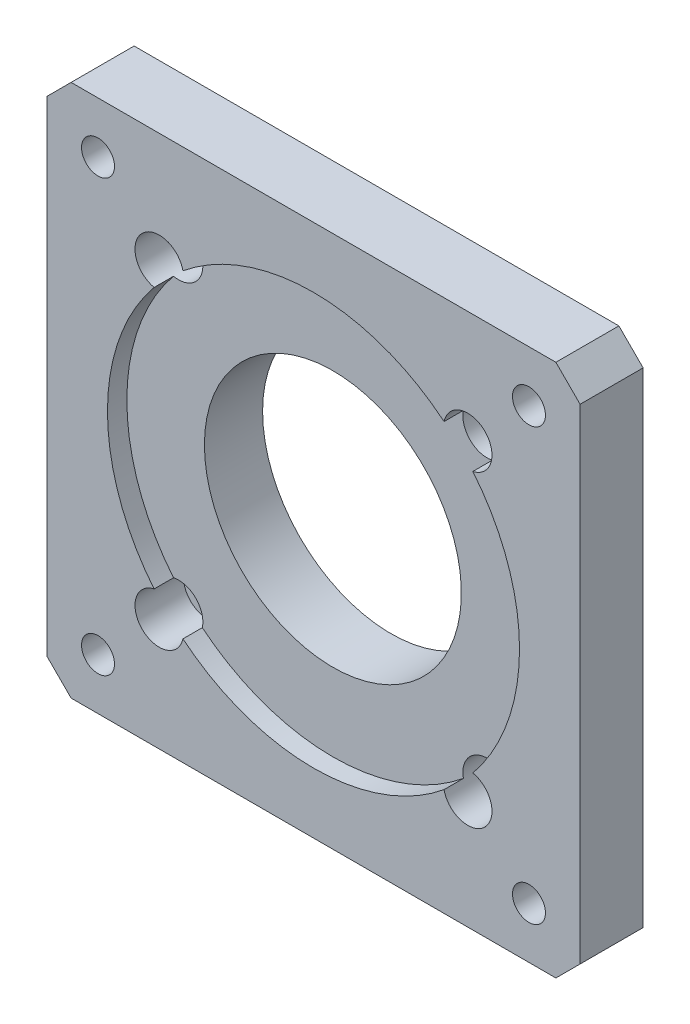
SolidWorks part; units mm, degrees
material "6061Al"
ref_plane "前视基准面" through (0, 0, 0) normal (0, 0, 1) x (1, 0, 0)
ref_plane "上视基准面" through (0, 0, 0) normal (0, 1, 0) x (1, 0, 0)
ref_plane "右视基准面" through (0, 0, 0) normal (1, 0, 0) x (0, 0, -1)
sketch "草图1" plane through (0, 0, 0) normal (0, 0, 1) x (1, 0, 0)
  line L1 (-55, 55) -> (55, 55)
  line L2 (-55, 55) -> (-55, -55)
  line L3 (-55, -55) -> (55, -55)
  line L4 (55, 55) -> (55, -55)
  line L5 (-55, 55) -> (55, -55) construction
  line L6 (-55, -55) -> (55, 55) construction
  point P0 (0, 0)
  dimension "D1" = 110
  dimension "D2" = 110
extrude "凸台-拉伸1" add sketch "草图1" along normal blind 13
sketch "草图2" plane through (0, 0, 13) normal (0, 0, 1) x (1, 0, 0)
  circle A0 centre (0, 0) radius 42.5
  dimension "D1" = 85
extrude "切除-拉伸1" cut sketch "草图2" against normal blind 4
sketch "草图3" plane through (0, 0, 0) normal (0, 0, -1) x (-1, 0, 0)
  circle A0 centre (0, 0) radius 26.5
  dimension "D1" = 53
extrude "切除-拉伸2" cut sketch "草图3" against normal through all
sketch "草图4" plane through (0, 0, 0) normal (0, 0, -1) x (-1, 0, 0)
  circle A0 centre (0, 0) radius 26.5 construction
  circle A1 centre (0, 0) radius 26.5
  circle A2 centre (0, 0) radius 35
  dimension "D1" = 70
extrude "凸台-拉伸2" add sketch "草图4" along normal blind 3
hole_wizard "M8 螺纹孔1" positions "草图5" profile "草图6" tap size "M8" standard "ISO" end condition through all
sketch "草图5" plane through (0, 0, 0) normal (0, 0, -1) x (-1, 0, 0)
  line L0 (0, 0) -> (-77.6797, 0) construction
  line L2 (0, 0) -> (0, 79.9272) construction
  point P0 (-44.45, 44.45)
  point P3 (44.45, 44.45)
  point P6 (44.45, -44.45)
  point P9 (-44.45, -44.45)
sketch "草图6" plane through (44.45, 44.45, 0) normal (1, 0, 0) x (0, 1, 0)
  line L0 (0, 0) -> (0, 13)
  line L1 (0, 13) -> (3.4, 13)
  line L2 (3.4, 13) -> (3.4, 0)
  line L5 (3.4, 0) -> (0, 0)
  line L11 (0, -6.35) -> (0, 107.95) construction
  dimension "通孔螺纹孔钻头直径" = 6.8
  dimension "通孔螺纹孔钻头深度" = 13
cosmetic thread "孔螺蚊线1" parameters "D2"=8
cosmetic thread "孔螺蚊线2" parameters "D2"=8
cosmetic thread "孔螺蚊线3" parameters "D2"=8
cosmetic thread "孔螺蚊线4" parameters "D2"=8
chamfer "倒角1" distance 5 angle 45 4 edges at (55, -55, 6.5) (-55, -55, 6.5) (-55, 55, 6.5) (55, 55, 6.5)
hole_wizard "M5 六角凹头螺钉的柱形沉头孔1" positions "草图7" profile "草图8" counterbore size "M5" standard "ISO" end condition through all
sketch "草图7" plane through (0, 0, 13) normal (0, 0, 1) x (1, 0, 0)
  point P0 (-31.8198, 31.8198)
  point P3 (-31.8198, -31.8198)
  point P6 (31.8198, -31.8198)
  point P9 (31.8198, 31.8198)
sketch "草图8" plane through (-31.8198, 31.8198, 13) normal (1, 0, 0) x (0, -1, 0)
  line L0 (0, 0) -> (0, 16)
  line L1 (0, 16) -> (2.9, 16)
  line L3 (2.9, 16) -> (2.9, 10)
  line L4 (2.9, 10) -> (5, 10)
  line L5 (5, 10) -> (5, 0)
  line L7 (5, 0) -> (0, 0)
  line L11 (0, -6.35) -> (0, 107.95) construction
  dimension "通孔孔直径" = 5.8
  dimension "通孔孔深度" = 16
  dimension "柱形沉头孔直径" = 10
  dimension "柱形沉头孔深度" = 10
chamfer "倒角2" distance 0.5 angle 45 1 edges at (-35, 0, -3)
equation "\"D2@草图5\"=\"D1@草图5\""
